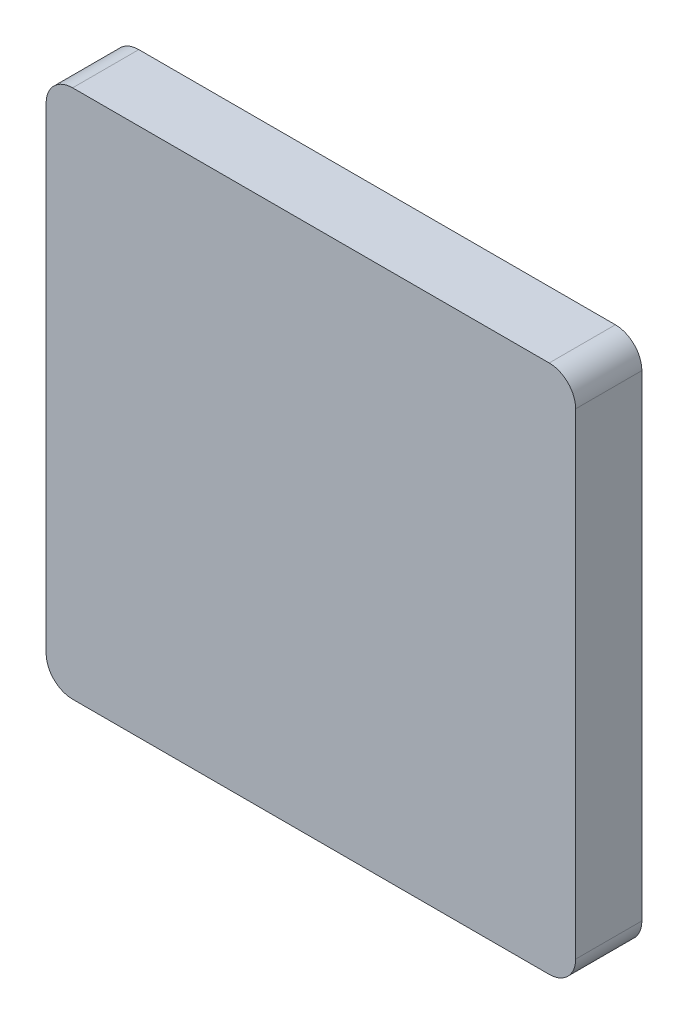
SolidWorks part; units mm, degrees
ref_plane "Front Plane" through (0, 0, 0) normal (0, 0, 1) x (1, 0, 0)
ref_plane "Top Plane" through (0, 0, 0) normal (0, 1, 0) x (1, 0, 0)
ref_plane "Right Plane" through (0, 0, 0) normal (1, 0, 0) x (0, 0, -1)
sketch "Sketch1" plane through (0, 0, 0) normal (0, 0, 1) x (1, 0, 0)
  line L1 (2, 0) -> (38, 0)
  line L2 (0, 2) -> (0, 38)
  line L3 (2, 40) -> (38, 40)
  line L4 (40, 2) -> (40, 38)
  arc A0 (2, 0) -> (0, 2) centre (2, 2) cw
  arc A1 (40, 2) -> (38, 0) centre (38, 2) cw
  arc A2 (40, 38) -> (38, 40) centre (38, 38) ccw
  arc A4 (0, 38) -> (2, 40) centre (2, 38) cw
  point P7 (40, 0)
  point P10 (0, 0)
  point P13 (0, 40)
  dimension "D3" = 2
  dimension "D4" = 2
  dimension "D1" = 40
  dimension "D2" = 40
extrude "Boss-Extrude1" add sketch "Sketch1" along normal blind 5
